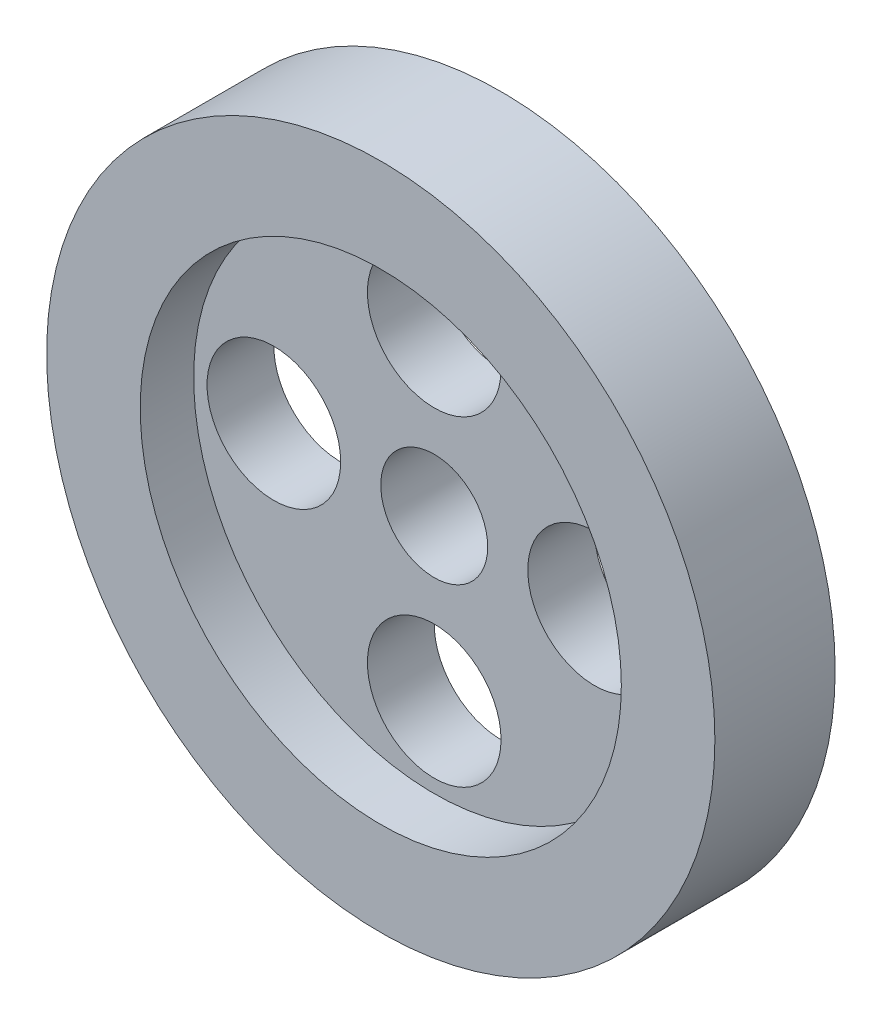
from build123d import *

# Parameters (mm, degrees)
SKETCH1_R           = 25
BOSS_EXTRUDE1_DEPTH = 9
SKETCH2_R           = 18
CUT_EXTRUDE1_DEPTH  = 4
SKETCH3_R           = 5
CUT_EXTRUDE2_DEPTH  = 36.707142143
SKETCH4_R           = 4
CUT_EXTRUDE3_DEPTH  = 36.707142143
SKETCH5_R           = 6
SKETCH5_R_2         = 4
BOSS_EXTRUDE2_DEPTH = 1


with BuildPart() as part:
    # Sketch1 → Boss-Extrude1 (new body)
    with BuildSketch(Plane.XY):
        Circle(SKETCH1_R)
    extrude(amount=BOSS_EXTRUDE1_DEPTH)

    # Sketch2 → Cut-Extrude1 (cut)
    with BuildSketch(Plane.XY.offset(9)):
        Circle(SKETCH2_R)
    extrude(amount=-CUT_EXTRUDE1_DEPTH, mode=Mode.SUBTRACT)

    # Sketch3 → Cut-Extrude2 (cut, through all)
    with BuildSketch(Plane.XY.offset(5)):
        with Locations((0, 12)):
            Circle(SKETCH3_R)
        with Locations((12, 0)):
            Circle(SKETCH3_R)
        with Locations((0, -12)):
            Circle(SKETCH3_R)
        with Locations((-12, 0)):
            Circle(SKETCH3_R)
    extrude(amount=-CUT_EXTRUDE2_DEPTH, mode=Mode.SUBTRACT)

    # Sketch4 → Cut-Extrude3 (cut, through all)
    with BuildSketch(Plane.XY.offset(5)):
        Circle(SKETCH4_R)
    extrude(amount=-CUT_EXTRUDE3_DEPTH, mode=Mode.SUBTRACT)

    # Sketch5 → Boss-Extrude2 (add)
    with BuildSketch(Plane(origin=(0, 0, 0), x_dir=(-1, 0, 0), z_dir=(0, 0, -1))):
        with Locations(Location((0, 0, 0), (0, 0, 180))):
            Circle(SKETCH5_R)
        with Locations(Location((0, 0, 0), (0, 0, 180))):
            Circle(SKETCH5_R_2, mode=Mode.SUBTRACT)
    extrude(amount=BOSS_EXTRUDE2_DEPTH)


solid = part.part
